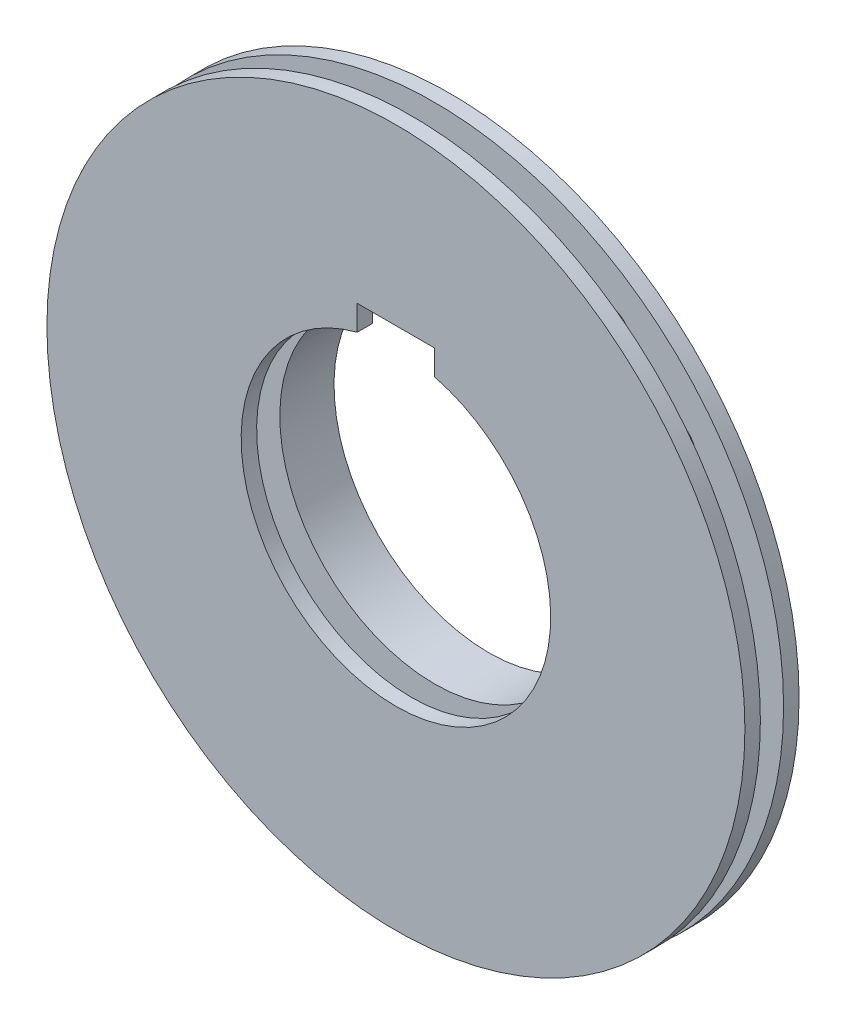
SolidWorks part; units mm, degrees
ref_plane "Front Plane" through (0, 0, 0) normal (0, 0, 1) x (1, 0, 0)
ref_plane "Top Plane" through (0, 0, 0) normal (0, 1, 0) x (1, 0, 0)
ref_plane "Right Plane" through (0, 0, 0) normal (1, 0, 0) x (0, 0, -1)
sketch "Sketch1" plane through (0, 0, 0) normal (0, 0, 1) x (1, 0, 0)
  circle A0 centre (0, 0) radius 100
  circle A1 centre (0, 0) radius 225.5
  dimension "D1" = 200
  dimension "D2" = 451
extrude "Boss-Extrude1" add sketch "Sketch1" along normal blind 10 from offset 7.5
mirror "Mirror1" about plane through (0, 0, 0) normal (0, 0, 1) of bodies 106
sketch "Sketch2" plane through (0, 0, -7.5) normal (0, 0, 1) x (1, 0, 0)
  circle A0 centre (0, 190) radius 15
  circle A2 centre (58.7132, 180.7007) radius 15
  circle A3 centre (111.6792, 153.7132) radius 15
  circle A4 centre (153.7132, 111.6792) radius 15
  circle A5 centre (180.7007, 58.7132) radius 15
  circle A6 centre (190, 0) radius 15
  circle A7 centre (180.7007, -58.7132) radius 15
  circle A8 centre (153.7132, -111.6792) radius 15
  circle A9 centre (111.6792, -153.7132) radius 15
  circle A10 centre (58.7132, -180.7007) radius 15
  circle A11 centre (0, -190) radius 15
  circle A12 centre (-58.7132, -180.7007) radius 15
  circle A13 centre (-111.6792, -153.7132) radius 15
  circle A14 centre (-153.7132, -111.6792) radius 15
  circle A15 centre (-180.7007, -58.7132) radius 15
  circle A16 centre (-190, 0) radius 15
  circle A17 centre (-180.7007, 58.7132) radius 15
  circle A18 centre (-153.7132, 111.6792) radius 15
  circle A19 centre (-111.6792, 153.7132) radius 15
  circle A20 centre (-58.7132, 180.7007) radius 15
  point P43 (0, 0)
  dimension "D1" = 30
  dimension "D2" = 190
  dimension "D3" = 20
extrude "Boss-Extrude2" add sketch "Sketch2" along normal up to surface (15 mm away) up to face at (225.5, 0, 7.5)
sketch "Sketch3" plane through (0, 0, 17.5) normal (0, 0, 1) x (1, 0, 0)
  line L1 (-25, 113) -> (25, 113)
  line L2 (-25, 113) -> (-25, 64.4044)
  line L3 (-25, 64.4044) -> (25, 64.4044)
  line L4 (25, 113) -> (25, 64.4044)
  dimension "D1" = 50
  dimension "D2" = 25
  dimension "D3" = 64.4044
  dimension "D4" = 113
extrude "Cut-Extrude1" cut sketch "Sketch3" against normal through all
sketch "Sketch4" plane through (0, 0, -17.5) normal (0, 0, -1) x (-1, 0, 0)
  line L0 (-25, 113) -> (25, 113) construction
  line L1 (25, 113) -> (25, 96.8246) construction
  line L2 (-25, 96.8246) -> (-25, 113) construction
  line L3 (-25, 113) -> (25, 113)
  line L4 (25, 113) -> (25, 96.8246)
  line L5 (-25, 96.8246) -> (-25, 113)
  arc A0 (-25, 96.8246) -> (25, 96.8246) centre (0, 0) ccw construction
  arc A1 (-25, 96.8246) -> (25, 96.8246) centre (0, 0) ccw
  circle A2 centre (0, 0) radius 130
  dimension "D1" = 260
extrude "Boss-Extrude3" add sketch "Sketch4" along normal blind 25
